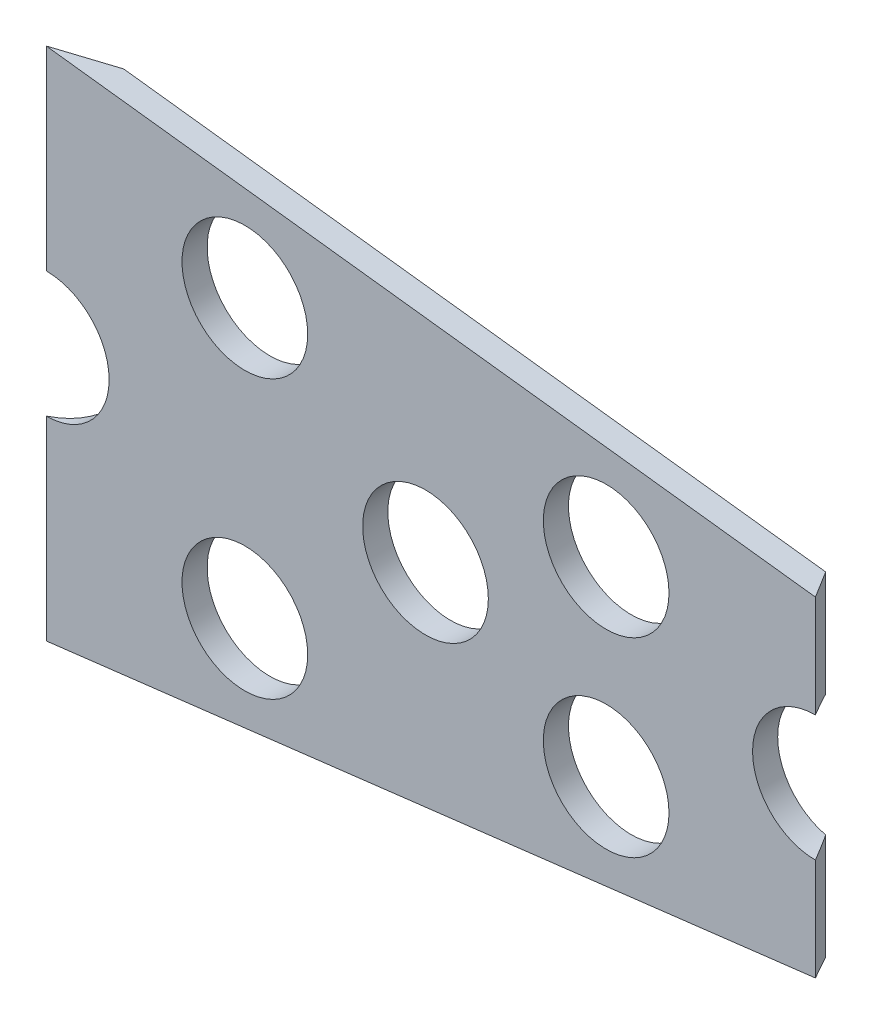
SolidWorks part; units mm, degrees
ref_plane "Front Plane" through (0, 0, 0) normal (0, 0, 1) x (1, 0, 0)
ref_plane "Top Plane" through (0, 0, 0) normal (0, 1, 0) x (1, 0, 0)
ref_plane "Right Plane" through (0, 0, 0) normal (1, 0, 0) x (0, 0, -1)
sketch "Sketch1" plane through (0, 0, 0) normal (0, 0, 1) x (1, 0, 0)
  line L0 (0, 0) -> (640.1463, 0) construction
  line L1 (0, 40) -> (0, 164)
  line L2 (489.6, 105) -> (489.6, 40)
  line L3 (0, 164) -> (489.6, 105)
  line L4 (241.4, 254.3602) -> (241.4, -154.9219) construction
  line L5 (60, 96.3355) -> (429.6, 51.7963) construction
  line L6 (126.4, 222.6182) -> (126.4, -191.3421) construction
  line L7 (60, 0) -> (60, 96.3355) construction
  line L8 (429.6, 51.7963) -> (429.6, 0) construction
  line L9 (356.4, 234.9291) -> (356.4, -165) construction
  line L10 (489.6, -105) -> (489.6, -40)
  line L11 (0, -164) -> (489.6, -105)
  line L12 (0, -40) -> (0, -164)
  line L13 (60, -96.3355) -> (429.6, -51.7963) construction
  line L15 (0, 0) -> (0, 164) construction
  line L16 (489.6, 105) -> (489.6, 0) construction
  circle A0 centre (241.4, 0) radius 40
  circle A1 centre (126.4, 88.3339) radius 40
  circle A2 centre (356.4, 60.6174) radius 40
  circle A3 centre (126.4, -88.3339) radius 40
  circle A4 centre (356.4, -60.6174) radius 40
  arc A5 (0, -40) -> (0, 40) centre (0, 0) ccw
  arc A6 (489.6, 40) -> (489.6, -40) centre (489.6, 0) ccw
  dimension "D8" = 80
  dimension "D9" = 80
  dimension "D10" = 80
  dimension "D11" = 80
  dimension "D12" = 80
  dimension "D13" = 80
  dimension "D14" = 80
  dimension "D1" = 328
  dimension "D2" = 489.6
  dimension "D3" = 210
  dimension "D5" = 482.8
  dimension "D6" = 115
  dimension "D7" = 115
  dimension "D15" = 489.6
  dimension "D4" = 60
extrude "Boss-Extrude1" add sketch "Sketch1" along normal blind 16
sketch "Sketch3" plane through (19.4802, -161.6525, 0) normal (0.1196, -0.9928, 0) x (0.9928, 0.1196, 0)
  line L0 (473.521, 16) -> (464.021, 0)
  line L1 (-19.6211, 0) -> (473.521, 0) construction
  line L2 (473.521, 16) -> (473.521, 0) construction
  line L3 (473.521, 16) -> (473.521, 0)
  line L5 (-19.6211, 16) -> (-19.6211, 0) construction
  line L6 (-19.6211, 16) -> (-19.6211, 0)
  line L7 (-19.6211, 0) -> (13.8789, 0)
  line L8 (-19.6211, 16) -> (13.8789, 0)
  line L9 (464.021, 0) -> (473.521, 0)
  dimension "D1" = 9.5
  dimension "D2" = 33.5
extrude "Cut-Extrude2" cut sketch "Sketch3" along direction (0, 1, 0) on the side against the normal blind 500
